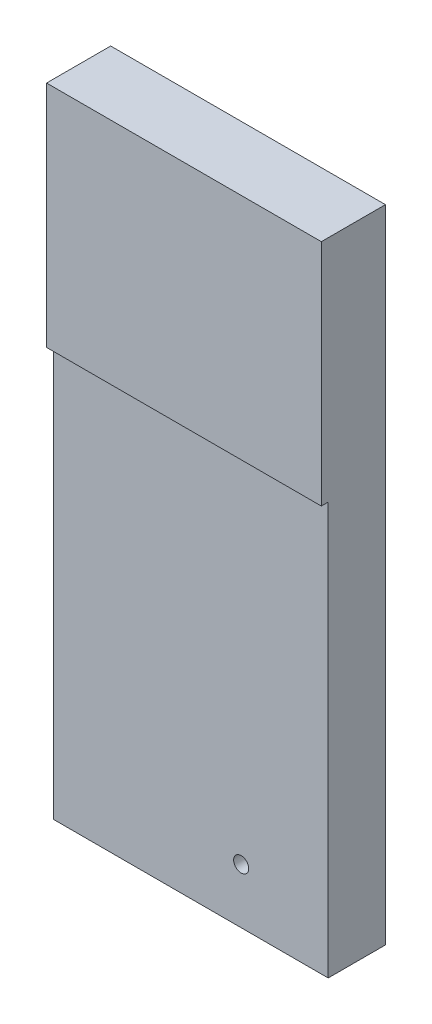
from build123d import *

# Parameters (mm, degrees)
SKETCH_1_W          = 60
SKETCH_1_H          = 140
EXTRUDE_1_DEPTH     = 14
SKETCH_2_W          = 60
SKETCH_2_H          = 90
CUT_EXTRUDE_1_DEPTH = 1.5
HOLE_WIZARD_M4_1_D  = 3.3


with BuildPart() as part:
    # 草图1 → 凸台-拉伸1 (new body)
    with BuildSketch(Plane.XY):
        Rectangle(SKETCH_1_W, SKETCH_1_H)
    extrude(amount=EXTRUDE_1_DEPTH)

    # 草图2 → 切除-拉伸1 (cut)
    with BuildSketch(Plane.XY.offset(14)):
        with Locations((0, -25)):
            Rectangle(SKETCH_2_W, SKETCH_2_H)
    extrude(amount=-CUT_EXTRUDE_1_DEPTH, mode=Mode.SUBTRACT)

    # M4 螺纹孔1 (through all)
    with Locations(Plane(origin=(0, 0, 0), x_dir=(-1, 0, 0), z_dir=(0, 0, -1))):
        with Locations((-11, -58)):
            Hole(HOLE_WIZARD_M4_1_D / 2)


solid = part.part
